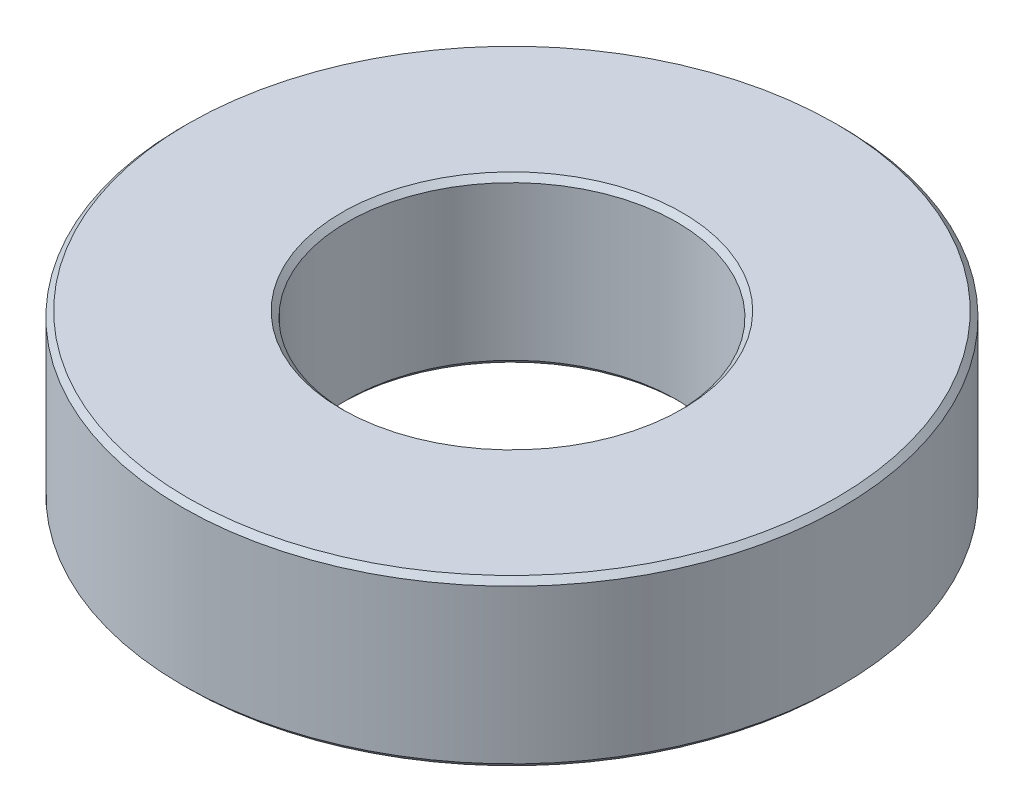
from build123d import *

# Parameters (mm, degrees)
SKETCH_1_R      = 12
SKETCH_1_R_2    = 6
EXTRUDE_1_DEPTH = 6
CHAMFER_1_SIZE  = 0.2


with BuildPart() as part:
    # 草图1 → 拉伸1 (new body)
    with BuildSketch(Plane(origin=(0, 0, 0), x_dir=(1, 0, 0), z_dir=(0, 1, 0))):
        with Locations(Location((0, 0, 0), (0, 0, 270))):
            Circle(SKETCH_1_R)
        with Locations(Location((0, 0, 0), (0, 0, 270))):
            Circle(SKETCH_1_R_2, mode=Mode.SUBTRACT)
    extrude(amount=EXTRUDE_1_DEPTH)

    # 倒角1
    chamfer_1_edges = [part.edges().sort_by_distance(p)[0] for p in [
        (0, 0, -12),
        (0, 6, -12),
        (0, 0, -6),
        (0, 6, -6),
    ]]
    chamfer(chamfer_1_edges, length=CHAMFER_1_SIZE)


solid = part.part
